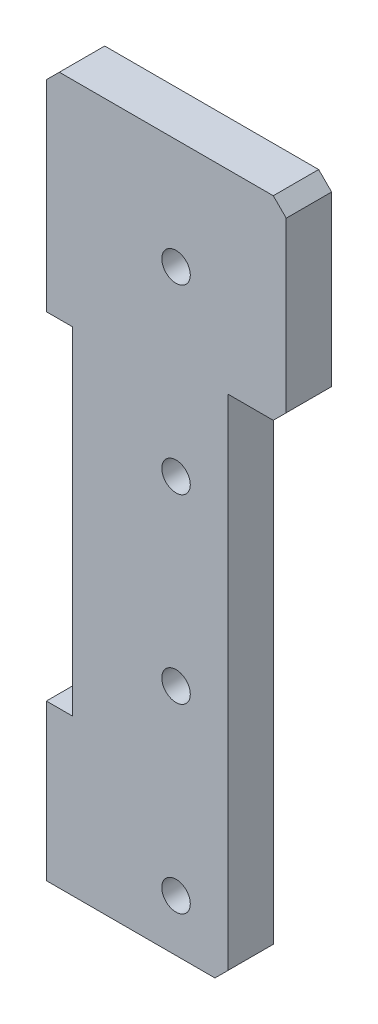
SolidWorks part; units mm, degrees
ref_plane "Front Plane" through (0, 0, 0) normal (0, 0, 1) x (1, 0, 0)
ref_plane "Top Plane" through (0, 0, 0) normal (0, 1, 0) x (1, 0, 0)
ref_plane "Right Plane" through (0, 0, 0) normal (1, 0, 0) x (0, 0, -1)
sketch "Sketch1" plane through (0, 0, 0) normal (0, 0, 1) x (1, 0, 0)
  line L1 (185, -150) -> (185, 0)
  line L2 (185, 0) -> (0, 0)
  line L3 (0, 0) -> (0, -165)
  line L4 (0, -165) -> (20, -165)
  line L6 (185, -150) -> (140, -150)
  line L7 (140, -150) -> (140, -545)
  line L8 (140, -545) -> (0, -545)
  line L9 (0, -545) -> (0, -425)
  line L10 (0, -425) -> (20, -425)
  line L11 (20, -425) -> (20, -165)
  dimension "D1" = 150
  dimension "D2" = 165
  dimension "D3" = 185
  dimension "D4" = 120
  dimension "D5" = 545
  dimension "D6" = 120
  dimension "D7" = 45
extrude "Boss-Extrude1" add sketch "Sketch1" along normal blind 35
chamfer "Chamfer1" distance 10 angle 45 4 edges at (140, -545, 17.5) (185, -150, 17.5) (0, 0, 17.5) (185, 0, 17.5)
sketch "Sketch2" plane through (0, 0, 35) normal (0, 0, 1) x (1, 0, 0)
  line L0 (185, -140) -> (185, -10) construction
  line L1 (140, -535) -> (140, -150) construction
  line L2 (175, 0) -> (10, 0) construction
  circle A0 centre (100, -85) radius 11
  circle A1 centre (100, -225) radius 11
  circle A2 centre (100, -365) radius 11
  circle A3 centre (100, -505) radius 11
  dimension "D9" = 22
  dimension "D1" = 85
  dimension "D2" = 40
  dimension "D3" = 40
  dimension "D4" = 40
  dimension "D5" = 85
  dimension "D6" = 140
  dimension "D7" = 140
  dimension "D8" = 140
extrude "Cut-Extrude1" cut sketch "Sketch2" against normal through all both and the other way through all
